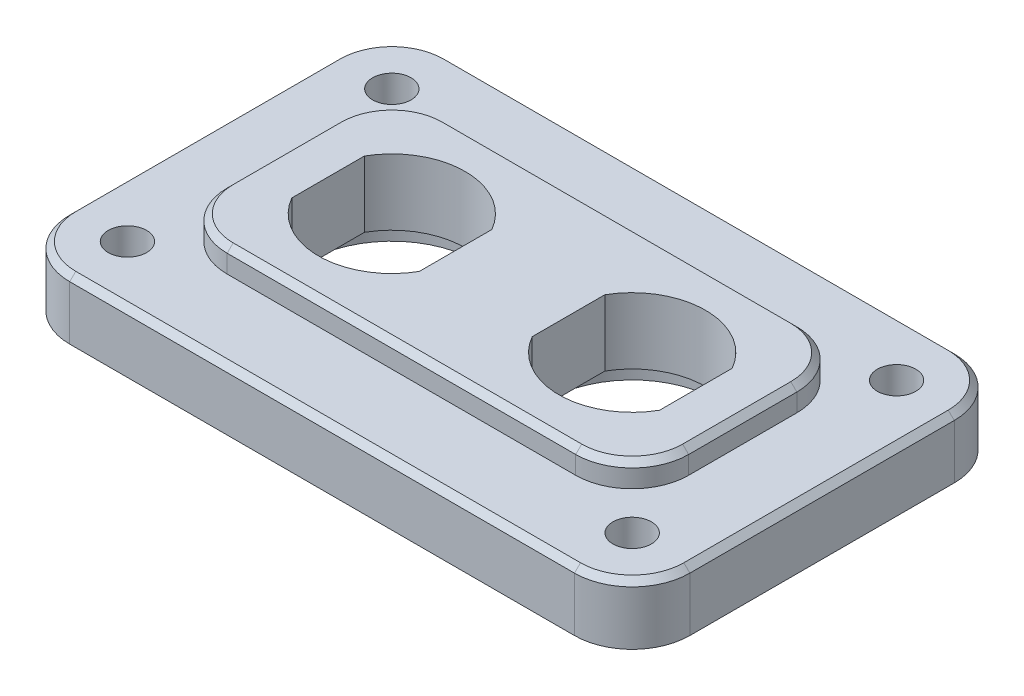
from build123d import *

# Parameters (mm, degrees)
SKETCH_1_W               = 31.6
SKETCH_1_H               = 5
EXTRUDE_1_DEPTH          = 25.8
EXTRUDE_2_DEPTH          = 2
FILLET_1_R               = 4.8
CUT_EXTRUDE_1_DEPTH      = 32.052858162
SKETCH_4_R               = 7.1
CUT_EXTRUDE_2_DEPTH      = 1.5
CHAMFER_2_SIZE           = 0.5
HOLE_WIZARD_1_AT_2_COUNT = 2
HOLE_WIZARD_1_AT_2_PITCH = 42
HOLE_WIZARD_1_AT_3_COUNT = 2
HOLE_WIZARD_1_AT_3_PITCH = 47.413078365
HOLE_WIZARD_1_AT_4_COUNT = 2
HOLE_WIZARD_1_AT_4_PITCH = 22


with BuildPart() as part:
    # 草图1 → 凸台-拉伸1 (new, symmetric)
    with BuildSketch(Plane(origin=(0, 0, 0), x_dir=(0, 0, -1), z_dir=(1, 0, 0))):
        with Locations((0, -2.5)):
            Rectangle(SKETCH_1_W, SKETCH_1_H)
    extrude(amount=EXTRUDE_1_DEPTH, both=True)

    # 草图2 → 凸台-拉伸2 (add)
    with BuildSketch(Plane(origin=(0, 0, 0), x_dir=(1, 0, 0), z_dir=(0, 1, 0))):
        with BuildLine():
            Line((-19.2, 4.5), (-19.2, -4.5))
            ThreePointArc((-19.2, -4.5), (-17.823401872, -7.823401872), (-14.5, -9.2))
            Line((-14.5, -9.2), (14.5, -9.2))
            ThreePointArc((14.5, -9.2), (17.823401872, -7.823401872), (19.2, -4.5))
            Line((19.2, -4.5), (19.2, 4.5))
            ThreePointArc((19.2, 4.5), (17.823401872, 7.823401872), (14.5, 9.2))
            Line((14.5, 9.2), (-14.5, 9.2))
            ThreePointArc((-14.5, 9.2), (-17.823401872, 7.823401872), (-19.2, 4.5))
        make_face()
    extrude(amount=EXTRUDE_2_DEPTH)

    # 圆角1
    fillet_1_edges = [part.edges().sort_by_distance(p)[0] for p in [
        (25.8, -2.5, 15.8),
        (25.8, -2.5, -15.8),
        (-25.8, -2.5, 15.8),
        (-25.8, -2.5, -15.8),
    ]]
    fillet(fillet_1_edges, radius=FILLET_1_R)

    # 草图3 → 切除-拉伸1 (cut, through all)
    with BuildSketch(Plane.XZ.offset(5)):
        with BuildLine():
            Line((-15.3, -3.019933774), (-15.3, 3.019933774))
            ThreePointArc((-15.3, 3.019933774), (-10, 6.1), (-4.7, 3.019933774))
            Line((-4.7, 3.019933774), (-4.7, -3.019933774))
            ThreePointArc((-4.7, -3.019933774), (-10, -6.1), (-15.3, -3.019933774))
        make_face()
        with BuildLine():
            Line((15.3, 3.019933774), (15.3, -3.019933774))
            ThreePointArc((15.3, -3.019933774), (10, -6.1), (4.7, -3.019933774))
            Line((4.7, -3.019933774), (4.7, 3.019933774))
            ThreePointArc((4.7, 3.019933774), (10, 6.1), (15.3, 3.019933774))
        make_face()
    extrude(amount=-CUT_EXTRUDE_1_DEPTH, mode=Mode.SUBTRACT)

    # 草图4 → 切除-拉伸2 (cut)
    with BuildSketch(Plane.XZ.offset(5)):
        with Locations(Location((-10, 0, 0), (0, 0, 270))):
            Circle(SKETCH_4_R)
        with Locations(Location((10, 0, 0), (0, 0, 270))):
            Circle(SKETCH_4_R)
    extrude(amount=-CUT_EXTRUDE_2_DEPTH, mode=Mode.SUBTRACT)

    # 倒角2
    chamfer_2_edges = [part.edges().sort_by_distance(p)[0] for p in [
        (17.823401872, 2, -7.823401872),
        (0, 2, -9.2),
        (-17.823401872, 2, -7.823401872),
        (-19.2, 2, 0),
        (-17.823401872, 2, 7.823401872),
        (0, 2, 9.2),
        (17.823401872, 2, 7.823401872),
        (19.2, 2, 0),
        (25.8, 0, 0),
        (-25.8, 0, 0),
        (0, 0, 15.8),
        (0, 0, -15.8),
        (-24.39411255, 0, 14.39411255),
        (-24.39411255, 0, -14.39411255),
        (24.39411255, 0, 14.39411255),
        (24.39411255, 0, -14.39411255),
    ]]
    chamfer(chamfer_2_edges, length=CHAMFER_2_SIZE)

    # 草图6 → 打孔尺寸(%根据十字)槽半沉头木螺钉的类型1 (revolve, cut)
    with BuildSketch(Plane(origin=(-21, -5, 11), x_dir=(0, 0, -1), z_dir=(1, 0, 0))):
        Polygon((0, 0), (0, 6.16137699), (1.6, 5.2), (1.6, 2.1), (3, 0.7), (3, 0), align=None)
    hole_wizard_1 = revolve(axis=Axis((-21, -11.35, 11), (0, 1, 0)), mode=Mode.SUBTRACT)

    # 打孔尺寸(%根据十字)槽半沉头木螺钉的类型1 at 2: 打孔尺寸(%根据十字)槽半沉头木螺钉的类型1 ×2
    with Locations(*[(i * HOLE_WIZARD_1_AT_2_PITCH, 0, 0) for i in range(1, HOLE_WIZARD_1_AT_2_COUNT)]):
        add(hole_wizard_1, mode=Mode.SUBTRACT)

    # 打孔尺寸(%根据十字)槽半沉头木螺钉的类型1 at 3: 打孔尺寸(%根据十字)槽半沉头木螺钉的类型1 ×2
    with Locations(*[Vector(0.8858315352801553, 0, -0.4640069946705578) * (i * HOLE_WIZARD_1_AT_3_PITCH) for i in range(1, HOLE_WIZARD_1_AT_3_COUNT)]):
        add(hole_wizard_1, mode=Mode.SUBTRACT)

    # 打孔尺寸(%根据十字)槽半沉头木螺钉的类型1 at 4: 打孔尺寸(%根据十字)槽半沉头木螺钉的类型1 ×2
    with Locations(*[(0, 0, -i * HOLE_WIZARD_1_AT_4_PITCH) for i in range(1, HOLE_WIZARD_1_AT_4_COUNT)]):
        add(hole_wizard_1, mode=Mode.SUBTRACT)


solid = part.part
